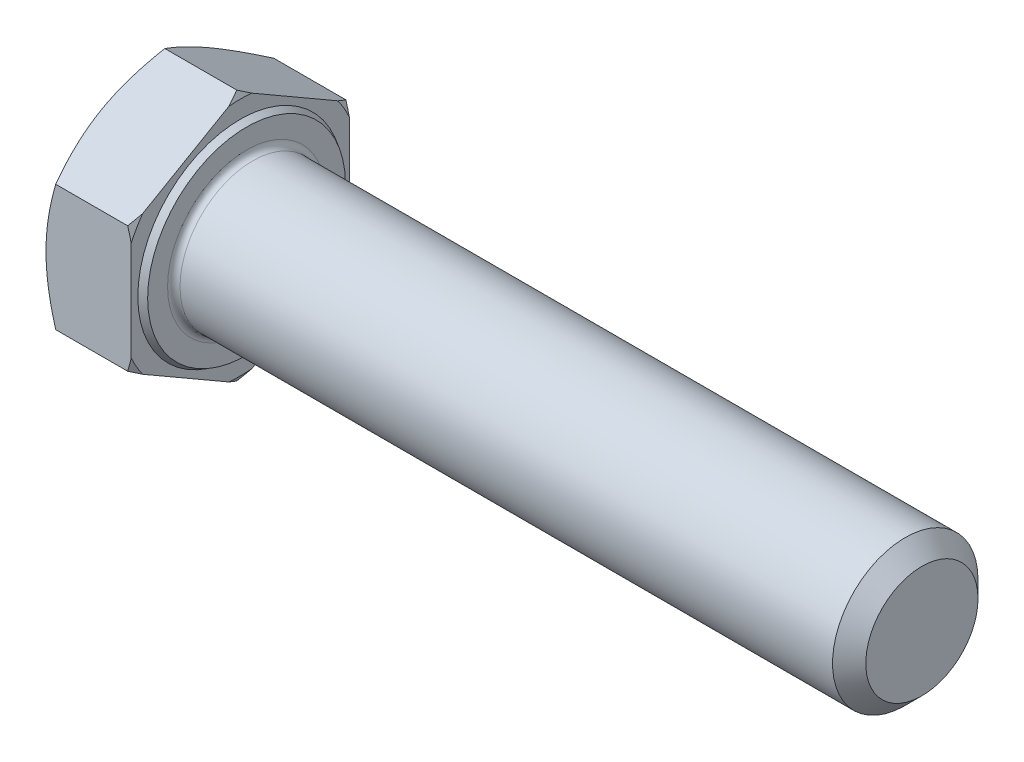
from build123d import *

# Parameters (mm, degrees)
BOSS_EXTRUDE_DEPTH = 8.8
CHAMFER_2_SIZE     = 1.6


with BuildPart() as part:
    # Sketch1 → Boss-Extrude (new body)
    with BuildSketch(Plane(origin=(0, 0, 0), x_dir=(0, 0, -1), z_dir=(1, 0, 0))):
        Polygon((10.5, 6.062177826), (10.5, -6.062177826), (0, -12.124355653), (-10.5, -6.062177826), (-10.5, 6.062177826), (0, 12.124355653), align=None)
    extrude(amount=BOSS_EXTRUDE_DEPTH)

    # Sketch2 → Boss-Revolve1 (revolve)
    with BuildSketch(Plane.XY, mode=Mode.PRIVATE) as boss_revolve1_sk:
        Polygon((0, 0), (73.8, 0), (73.8, 5.268), (73.8, 7), (8.8, 7), (0, 7), align=None)
    revolve(boss_revolve1_sk.sketch.rotate(Axis((0, 0, 0), (-1, 0, 0)), 90), axis=Axis((0, 0, 0), (-1, 0, 0)))

    # Sketch3 → Cut-Revolve1 (revolve, cut)
    with BuildSketch(Plane.XY):
        Polygon((0, 10.5), (3.824573519, 17.124355653), (3.824573519, 22.124355653), (-10, 22.124355653), (-10, 10.5), align=None)
    revolve(axis=Axis((0, 0, 0), (1, 0, 0)), mode=Mode.SUBTRACT)

    # Sketch5 → Cut-Revolve2 (revolve, cut)
    with BuildSketch(Plane.XY):
        Polygon((8.8, 10.5), (4.975426481, 17.124355653), (4.975426481, 22.124355653), (14.975426481, 22.124355653), (14.975426481, 10.5), align=None)
    revolve(axis=Axis((0, 0, 0), (1, 0, 0)), mode=Mode.SUBTRACT)

    # Sketch4 → Cut-Revolve3 (revolve, cut)
    with BuildSketch(Plane.XY, mode=Mode.PRIVATE) as cut_revolve3_sk:
        Polygon((8.8, 9.517264973), (8.2, 9.863675135), (8.2, 22.124355653), (8.8, 22.124355653), align=None)
    revolve(cut_revolve3_sk.sketch.rotate(Axis((0, 0, 0), (1, 0, 0)), 90), axis=Axis((0, 0, 0), (1, 0, 0)), mode=Mode.SUBTRACT)

    # Chamfer 2
    chamfer_2_edges = [part.edges().sort_by_distance(p)[0] for p in [
        (73.8, 0, 7),
    ]]
    chamfer(chamfer_2_edges, length=CHAMFER_2_SIZE)

    # Sketch9 → Revolve1 (revolve)
    with BuildSketch(Plane.XY, mode=Mode.PRIVATE) as revolve1_sk:
        with BuildLine():
            Line((8.8, 7.6), (8.8, 7))
            Line((8.8, 7), (9.4, 7))
            ThreePointArc((9.4, 7), (8.975735931, 7.175735931), (8.8, 7.6))
        make_face()
    revolve(revolve1_sk.sketch.rotate(Axis((0, 0, 0), (1, 0, 0)), 90), axis=Axis((0, 0, 0), (1, 0, 0)))


solid = part.part
